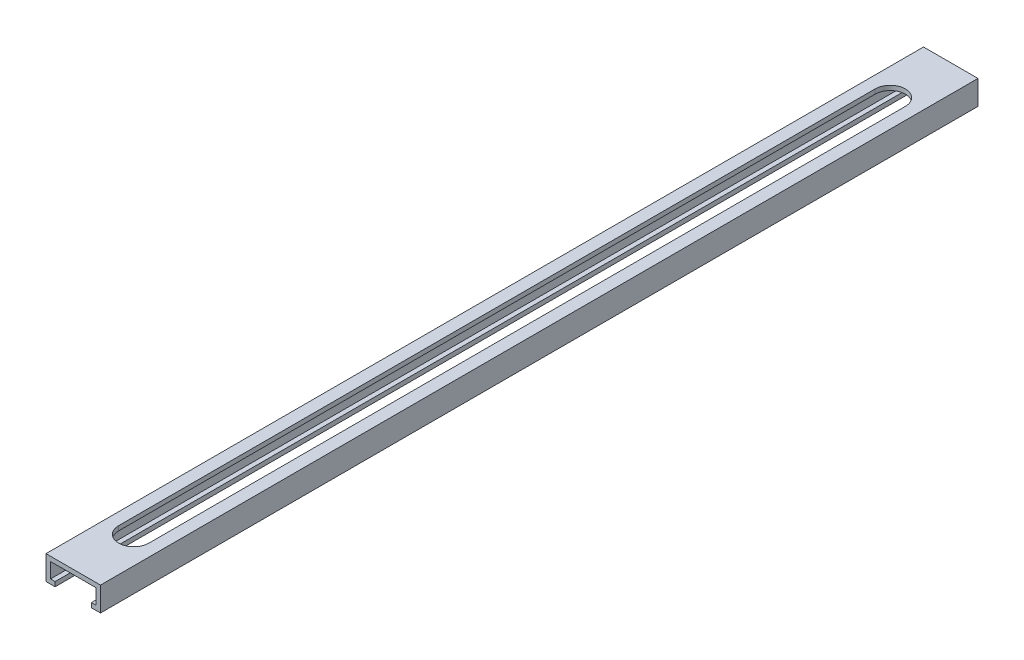
from build123d import *

# Parameters (mm, degrees)
SKETCH1_W           = 36
SKETCH1_H           = 580
BOSS_EXTRUDE1_DEPTH = 16
CUT_EXTRUDE1_DEPTH  = 581.424844403
CUT_EXTRUDE2_DEPTH  = 291.848757948


with BuildPart() as part:
    # Sketch1 → Boss-Extrude1 (new body)
    with BuildSketch(Plane(origin=(0, 13, 0), x_dir=(1, 0, 0), z_dir=(0, 1, 0))):
        Rectangle(SKETCH1_W, SKETCH1_H)
    extrude(amount=-BOSS_EXTRUDE1_DEPTH)

    # Sketch2 → Cut-Extrude1 (cut, through all)
    with BuildSketch(Plane(origin=(0, 0, -290), x_dir=(-1, 0, 0), z_dir=(0, 0, -1))):
        Polygon((12, -3), (12, 0), (15, 0), (15, 10), (-15, 10), (-15, 0), (-12, 0), (-12, -3), align=None)
    extrude(amount=-CUT_EXTRUDE1_DEPTH, mode=Mode.SUBTRACT)

    # Sketch3 → Cut-Extrude2 (cut, through all)
    with BuildSketch(Plane.XZ.offset(-10)):
        with BuildLine():
            Line((10, -250), (10, 250))
            ThreePointArc((10, 250), (0, 260), (-10, 250))
            Line((-10, 250), (-10, -250))
            ThreePointArc((-10, -250), (0, -260), (10, -250))
        make_face()
    extrude(amount=-CUT_EXTRUDE2_DEPTH, mode=Mode.SUBTRACT)


solid = part.part
